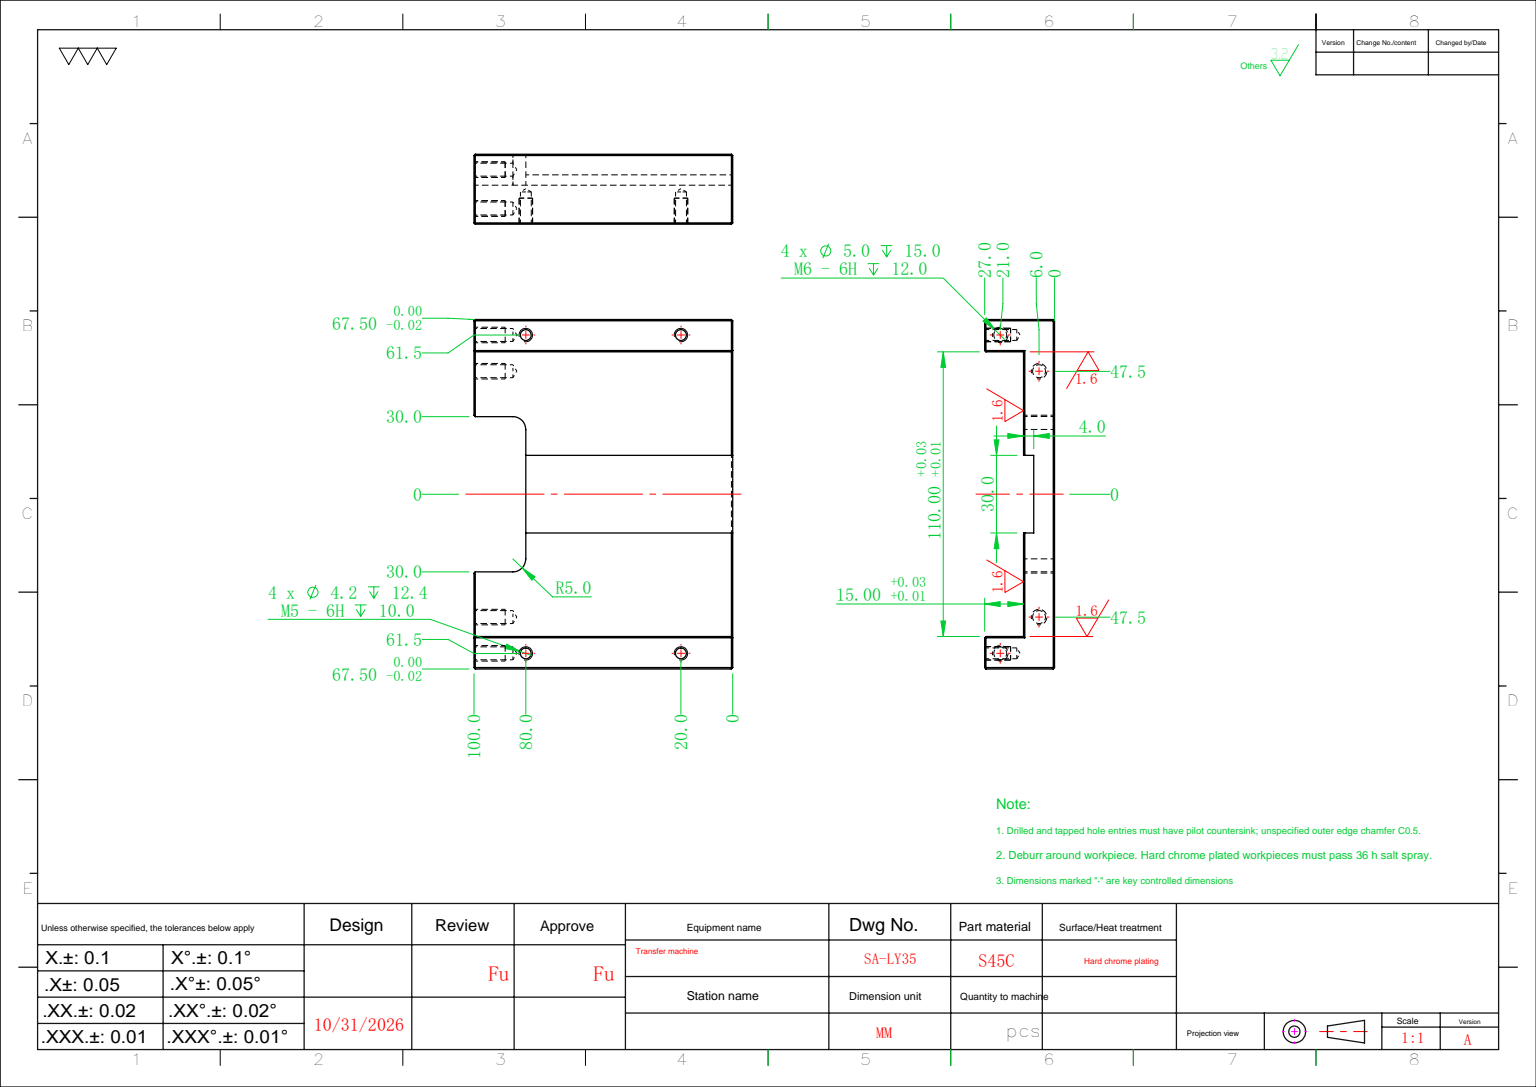
from build123d import *

# Parameters (mm, degrees)
SKETCH_1_W             = 135
SKETCH_1_H             = 100
EXTRUDE_1_DEPTH        = 12
SKETCH_2_W             = 12.5
SKETCH_2_H             = 100
EXTRUDE_2_DEPTH        = 15
SKETCH_3_W             = 30
SKETCH_3_H             = 200
CUT_EXTRUDE_1_DEPTH    = 4
SKETCH_4_W             = 60
SKETCH_4_H             = 20
CUT_EXTRUDE_2_DEPTH    = 86.330240829
FILLET_1_R             = 5
HOLE_WIZARD_M6_1_D     = 5
HOLE_WIZARD_M6_1_DEPTH = 15
HOLE_WIZARD_M6_1_TIP   = 1.502151548
HOLE_WIZARD_M5_1_D     = 4.2
HOLE_WIZARD_M5_1_DEPTH = 12.4
HOLE_WIZARD_M5_1_TIP   = 1.2618073
CHAMFER_1_SIZE         = 0.5


with BuildPart() as part:
    # 草图1 → 凸台-拉伸1 (new body)
    with BuildSketch(Plane.XY):
        Rectangle(SKETCH_1_W, SKETCH_1_H)
    extrude(amount=EXTRUDE_1_DEPTH)

    # 草图2 → 凸台-拉伸2 (add)
    with BuildSketch(Plane.XY.offset(12)):
        with Locations((-61.25, 0)):
            Rectangle(SKETCH_2_W, SKETCH_2_H)
        with Locations((61.25, 0)):
            Rectangle(SKETCH_2_W, SKETCH_2_H)
    extrude(amount=EXTRUDE_2_DEPTH)

    # 草图3 → 切除-拉伸1 (cut)
    with BuildSketch(Plane.XY.offset(12)):
        with Locations((0, 50)):
            Rectangle(SKETCH_3_W, SKETCH_3_H)
    extrude(amount=-CUT_EXTRUDE_1_DEPTH, mode=Mode.SUBTRACT)

    # 草图4 → 切除-拉伸2 (cut, through all)
    with BuildSketch(Plane.XY.offset(12)):
        with Locations((0, 40)):
            Rectangle(SKETCH_4_W, SKETCH_4_H)
    extrude(amount=-CUT_EXTRUDE_2_DEPTH, mode=Mode.SUBTRACT)

    # 圆角1
    fillet_1_edges = [part.edges().sort_by_distance(p)[0] for p in [
        (30, 30, 6),
        (-30, 30, 6),
    ]]
    fillet(fillet_1_edges, radius=FILLET_1_R)

    # M6 螺纹孔1
    with Locations(Plane(origin=(0, 50, 0), x_dir=(1, 0, 0), z_dir=(0, 1, 0))):
        with Locations((-61.5, -21), (-47.5, -6), (47.5, -6), (61.5, -21)):
            Hole(HOLE_WIZARD_M6_1_D / 2, depth=HOLE_WIZARD_M6_1_DEPTH)
            with Locations((0, 0, -(HOLE_WIZARD_M6_1_DEPTH + HOLE_WIZARD_M6_1_TIP / 2))):  # 118° drill point
                Cone(0, HOLE_WIZARD_M6_1_D / 2, HOLE_WIZARD_M6_1_TIP, mode=Mode.SUBTRACT)

    # M5 螺纹孔1
    with Locations(Plane.XY.offset(27)):
        with Locations((-61.5, 30), (-61.5, -30), (61.5, -30), (61.5, 30)):
            Hole(HOLE_WIZARD_M5_1_D / 2, depth=HOLE_WIZARD_M5_1_DEPTH)
            with Locations((0, 0, -(HOLE_WIZARD_M5_1_DEPTH + HOLE_WIZARD_M5_1_TIP / 2))):  # 118° drill point
                Cone(0, HOLE_WIZARD_M5_1_D / 2, HOLE_WIZARD_M5_1_TIP, mode=Mode.SUBTRACT)

    # 倒角1
    chamfer_1_edges = [part.edges().sort_by_distance(p)[0] for p in [
        (-35, -50, 12),
        (-55, -50, 19.5),
        (-55, 50, 19.5),
        (-67.5, 0, 27),
        (-61.25, -50, 27),
        (-55, 0, 27),
        (-61.25, 50, 27),
        (42.5, 50, 12),
        (55, 50, 19.5),
        (55, -50, 19.5),
        (61.25, 50, 27),
        (55, 0, 27),
        (61.25, -50, 27),
        (67.5, 0, 27),
        (35, -50, 12),
        (0, -50, 0),
        (-67.5, 0, 0),
        (48.75, 50, 0),
        (67.5, 0, 0),
        (-48.75, 50, 0),
        (-42.5, 50, 12),
        (-30, 50, 6),
        (30, 50, 6),
        (67.5, -50, 13.5),
        (-67.5, -50, 13.5),
        (-67.5, 50, 13.5),
        (67.5, 50, 13.5),
    ]]
    chamfer(chamfer_1_edges, length=CHAMFER_1_SIZE)


solid = part.part
